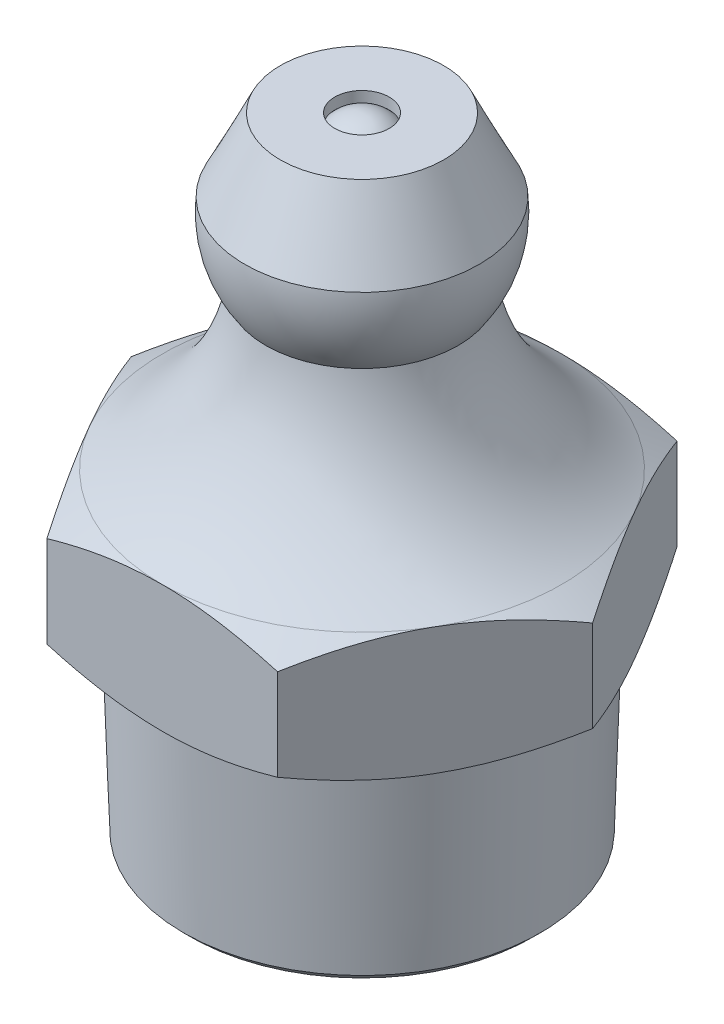
from build123d import *

# Parameters (mm, degrees)
EXTRUDE_START        = 9.5
EXTRUDE_1_DEPTH      = 3.5
CUT_EXTRUDE_START    = 9.5
SKETCH_3_3_OUTSIDE_W = 30.686
SKETCH_3_3_OUTSIDE_H = 28.984
SKETCH_3_3_OUTSIDE_R = 5.5
CUT_EXTRUDE_1_DEPTH  = 3.5
CUT_EXTRUDE_1_DRAFT  = -60
CUT_EXTRUDE_START_2  = 6
SKETCH_3_4_OUTSIDE_W = 30.686
SKETCH_3_4_OUTSIDE_H = 28.984
SKETCH_3_4_OUTSIDE_R = 5.5
CUT_EXTRUDE_2_DEPTH  = 3.5
CUT_EXTRUDE_2_DRAFT  = 60


with BuildPart() as part:
    # 草图2 → 旋转1 (revolve)
    with BuildSketch(Plane.XY, mode=Mode.PRIVATE) as revolve_1_sk:
        Polygon((0, 0), (-2.5, 0), (-2.5, 0.7), (-4.7125, 0.7), (-4.9125, 0.9), (-5.071875, 6), (-5.5, 6), (-5.5, 9.5), (0, 9.5), align=None)
    revolve(revolve_1_sk.sketch.rotate(Axis((0, 0, 0), (0, 1, 0)), 270), axis=Axis((0, 0, 0), (0, 1, 0)))

    # 草图3 → 凸台-拉伸1 (add)
    with BuildSketch(Plane(origin=(0, 0, 0), x_dir=(1, 0, 0), z_dir=(0, 1, 0)).offset(EXTRUDE_START)):
        Polygon((6.350852961, 0), (3.175426481, 5.5), (-3.175426481, 5.5), (-6.350852961, 0), (-3.175426481, -5.5), (3.175426481, -5.5), align=None)
    extrude(amount=-EXTRUDE_1_DEPTH)


with BuildPart() as cut_extrude_1_tool:
    # 草图3<3> outside → 切除-拉伸1 (with draft: the straight prism first)
    with BuildSketch(Plane(origin=(0, 0, 0), x_dir=(1, 0, 0), z_dir=(0, 1, 0)).offset(CUT_EXTRUDE_START)):
        Rectangle(SKETCH_3_3_OUTSIDE_W, SKETCH_3_3_OUTSIDE_H)
        Circle(SKETCH_3_3_OUTSIDE_R, mode=Mode.SUBTRACT)
    extrude(amount=-CUT_EXTRUDE_1_DEPTH)
    # 切除-拉伸1: the draft: its side faces are tilted about the plane it starts from
    cut_extrude_1_sides = [cut_extrude_1_tool.faces().sort_by_distance(p)[0] for p in [
        (0, 7.75, 14.492),
        (15.343, 7.75, 0),
        (0, 7.75, -14.492),
        (-15.343, 7.75, 0),
        (-5.5, 7.75, 0),
    ]]
    draft(cut_extrude_1_sides, Plane(origin=(0, 0, 0), x_dir=(1, 0, 0), z_dir=(0, 1, 0)).offset(CUT_EXTRUDE_START), CUT_EXTRUDE_1_DRAFT)


with BuildPart() as part_1:
    add(part.part)

    # 切除-拉伸1: cut by cut_extrude_1_tool
    add(cut_extrude_1_tool.part, mode=Mode.SUBTRACT)


with BuildPart() as cut_extrude_2_tool:
    # 草图3<4> outside → 切除-拉伸2 (with draft: the straight prism first)
    with BuildSketch(Plane(origin=(0, 0, 0), x_dir=(1, 0, 0), z_dir=(0, 1, 0)).offset(CUT_EXTRUDE_START_2)):
        Rectangle(SKETCH_3_4_OUTSIDE_W, SKETCH_3_4_OUTSIDE_H)
        Circle(SKETCH_3_4_OUTSIDE_R, mode=Mode.SUBTRACT)
    extrude(amount=CUT_EXTRUDE_2_DEPTH)
    # 切除-拉伸2: the draft: its side faces are tilted about the plane it starts from
    cut_extrude_2_sides = [cut_extrude_2_tool.faces().sort_by_distance(p)[0] for p in [
        (0, 7.75, 14.492),
        (15.343, 7.75, 0),
        (0, 7.75, -14.492),
        (-15.343, 7.75, 0),
        (-5.5, 7.75, 0),
    ]]
    draft(cut_extrude_2_sides, Plane(origin=(0, 0, 0), x_dir=(1, 0, 0), z_dir=(0, 1, 0)).offset(CUT_EXTRUDE_START_2), CUT_EXTRUDE_2_DRAFT)


with BuildPart() as part_2:
    add(part_1.part)

    # 切除-拉伸2: cut by cut_extrude_2_tool
    add(cut_extrude_2_tool.part, mode=Mode.SUBTRACT)

    # 草图4 → 旋转2 (revolve)
    with BuildSketch(Plane.XY, mode=Mode.PRIVATE) as revolve_2_sk:
        with BuildLine():
            Line((-0.75, 18), (-2.25, 18))
            Line((-2.25, 18), (-3.231614383, 16))
            ThreePointArc((-3.231614383, 16), (-3.144501778, 14.833446537), (-2.65, 13.773303348))
            ThreePointArc((-2.65, 13.773303348), (-3.602356761, 11.321431077), (-5.5, 9.5))
            Line((-5.5, 9.5), (-1.5, 9.5))
            Line((-1.5, 9.5), (-1.5, 16.939339828))
            Line((-1.5, 16.939339828), (-0.75, 17.689339828))
            Line((-0.75, 17.689339828), (-0.75, 18))
        make_face()
    revolve(revolve_2_sk.sketch.rotate(Axis((0, 18, 0), (0, -1, 0)), 270), axis=Axis((0, 18, 0), (0, -1, 0)))


with BuildPart() as body_2:
    # 草图5 → 旋转3 (revolve)
    with BuildSketch(Plane.XY):
        with BuildLine():
            Line((0, 15.878679656), (0, 18))
            ThreePointArc((0, 18), (-1.060660172, 16.939339828), (0, 15.878679656))
        make_face()
    revolve(axis=Axis((0, 0, 0), (0, 1, 0)))


solid = Compound([part_2.part, body_2.part])
